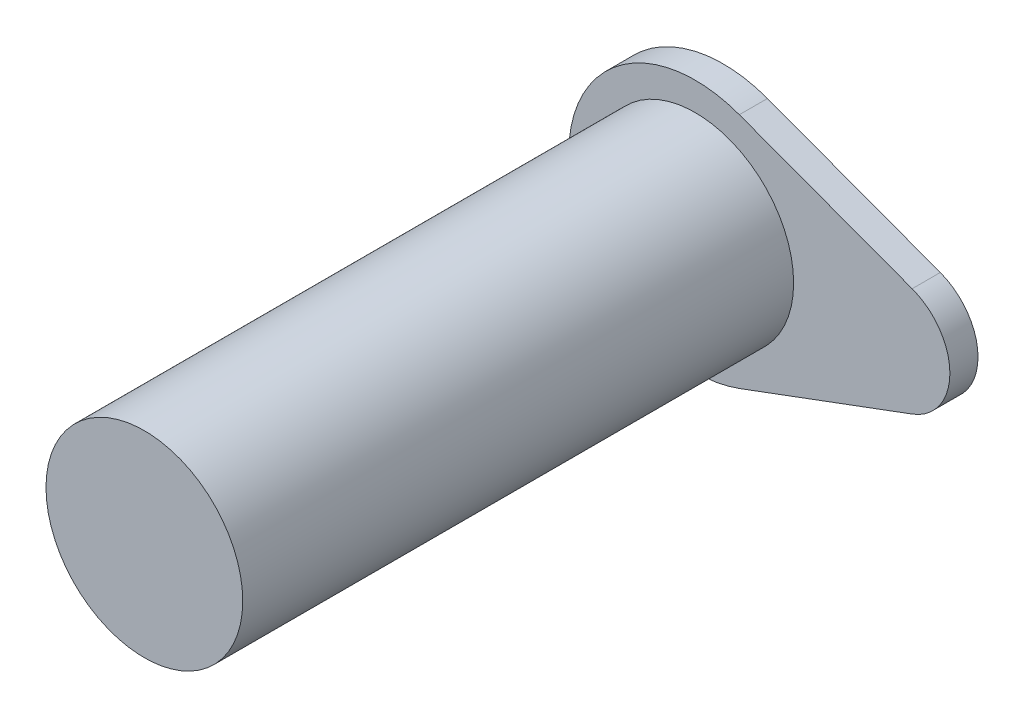
SolidWorks part; units mm, degrees
ref_plane "前视基准面" through (0, 0, 0) normal (0, 0, 1) x (1, 0, 0)
ref_plane "上视基准面" through (0, 0, 0) normal (0, 1, 0) x (1, 0, 0)
ref_plane "右视基准面" through (0, 0, 0) normal (1, 0, 0) x (0, 0, -1)
sketch "草图1" plane through (0, 0, 0) normal (0, 0, 1) x (1, 0, 0)
  circle A0 centre (0, 0) radius 17.5
extrude "凸台-拉伸1" add sketch "草图1" along normal blind 103
sketch "草图2" plane through (0, 0, 0) normal (0, 0, -1) x (-1, 0, 0)
  line L3 (-38.5903, 9.6552) -> (-7.8421, 21.0891)
  line L4 (-38.5903, -9.6552) -> (-7.8421, -21.0891)
  circle A2 centre (-35, 0) radius 10.3011
  arc A3 (-7.8421, -21.0891) -> (-7.8421, 21.0891) centre (0, 0) ccw
extrude "凸台-拉伸3" add sketch "草图2" against normal blind 5 contours L3 | A2 | L4 A3 L3 A2
sketch "草图3" plane through (0, 0, 0) normal (0, 0, -1) x (-1, 0, 0)
  circle A0 centre (0, 0) radius 4
extrude "切除-拉伸1" cut sketch "草图3" against normal blind 70
cosmetic thread "装饰螺纹线1" parameters "D1"=5, "D2"=9
sketch "草图4" plane through (0, 0, 0) normal (0, 1, 0) x (1, 0, 0)
  line L0 (0, -103) -> (0, 0)
  line L1 (-17.5, -103) -> (17.5, -103) construction
  line L2 (0, -51.5) -> (4, -51.5)
  circle A0 centre (0, -51.5) radius 4
extrude "切除-拉伸2" cut sketch "草图4" against normal blind 70 contours L2 A0 L0 | L0 A0 L2 | L0 A0
